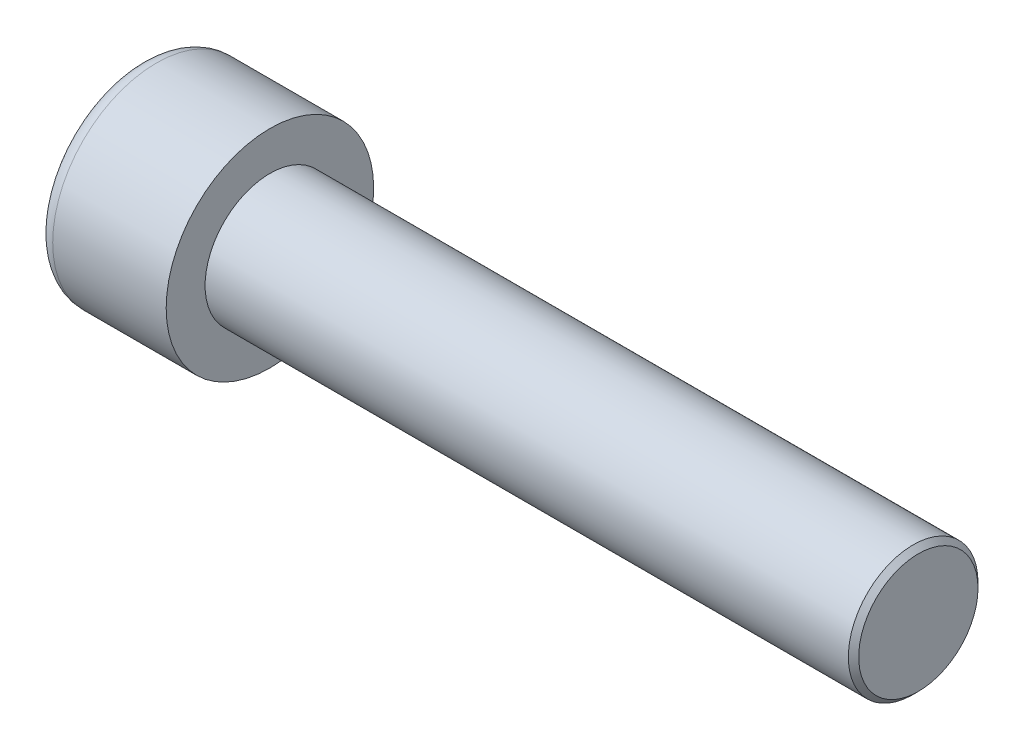
from build123d import *

# Parameters (mm, degrees)
SKETCH1_R           = 8
BASEHEAD_DEPTH      = 10
SKETCH2_R           = 5
BASEBODY_DEPTH      = 50
HEXAGONSOCKET_DEPTH = 5
TOPFILLET_R         = 1.25
CHAMFER1_SIZE       = 0.4


with BuildPart() as part:
    # Sketch1 → BaseHead (new body)
    with BuildSketch(Plane(origin=(0, 0, 0), x_dir=(0, 0, -1), z_dir=(1, 0, 0))):
        Circle(SKETCH1_R)
    extrude(amount=BASEHEAD_DEPTH)

    # Sketch2 → BaseBody (add)
    with BuildSketch(Plane(origin=(10, 0, 0), x_dir=(0, 0, -1), z_dir=(1, 0, 0))):
        Circle(SKETCH2_R)
    extrude(amount=BASEBODY_DEPTH)

    # Sketch3 → HexagonSocket (cut)
    with BuildSketch(Plane(origin=(0, 0, 0), x_dir=(0, 0, -1), z_dir=(1, 0, 0))):
        Polygon((4.618802154, 0), (2.309401077, 4), (-2.309401077, 4), (-4.618802154, 0), (-2.309401077, -4), (2.309401077, -4), align=None)
    extrude(amount=HEXAGONSOCKET_DEPTH, mode=Mode.SUBTRACT)

    # Sketch4 → Cut-Revolve1 (revolve, cut)
    with BuildSketch(Plane(origin=(-4.19613823, 0.75, 0), x_dir=(-1, 0, 0), z_dir=(0, 0, 1)), mode=Mode.PRIVATE) as cut_revolve1_sk:
        Polygon((-9.19613823, 4.75), (-11.505539306, 0.75), (-9.19613823, 0.75), align=None)
    revolve(cut_revolve1_sk.sketch.rotate(Axis((0.838992387, 0, 0), (-1, 0, 0)), 90), axis=Axis((0.838992387, 0, 0), (-1, 0, 0)), mode=Mode.SUBTRACT)

    # TopFillet
    topfillet_edges = [part.edges().sort_by_distance(p)[0] for p in [
        (0, 0, 8),
    ]]
    fillet(topfillet_edges, radius=TOPFILLET_R)

    # Chamfer1
    chamfer1_edges = [part.edges().sort_by_distance(p)[0] for p in [
        (60, 0, 5),
    ]]
    chamfer(chamfer1_edges, length=CHAMFER1_SIZE)


solid = part.part
